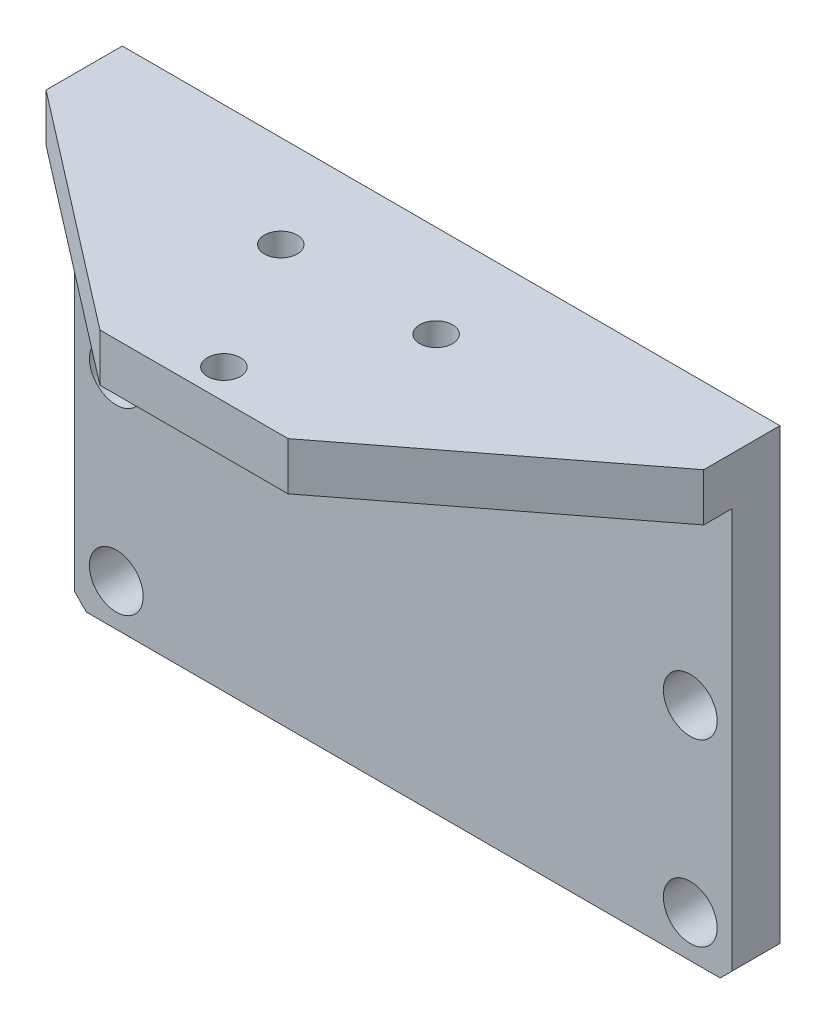
from build123d import *

# Parameters (mm, degrees)
SKETCH_1_W              = 110
SKETCH_1_H              = 77
EXTRUDE_1_DEPTH         = 8
SKETCH_2_W              = 110
SKETCH_2_H              = 8
EXTRUDE_3_DEPTH         = 43
SKETCH_4_OUTSIDE_W      = 140.198
SKETCH_4_OUTSIDE_H      = 73.198
CUT_EXTRUDE_1_DEPTH     = 43
HOLE_WIZARD_7_0_7_1_D   = 9
HOLE_WIZARD_5_5_5_5_2_D = 5.5
CHAMFER_1_SIZE          = 2


with BuildPart() as part:
    # 草图1 → 凸台-拉伸1 (new body)
    with BuildSketch(Plane.XY):
        Rectangle(SKETCH_1_W, SKETCH_1_H)
    extrude(amount=EXTRUDE_1_DEPTH)

    # 草图2 → 凸台-拉伸3 (add)
    with BuildSketch(Plane.XY):
        with Locations((0, 34.5)):
            Rectangle(SKETCH_2_W, SKETCH_2_H)
    extrude(amount=EXTRUDE_3_DEPTH)

    # 草图4 outside → 切除-拉伸1 (cut)
    with BuildSketch(Plane(origin=(0, 38.5, 0), x_dir=(1, 0, 0), z_dir=(0, 1, 0))):
        with Locations((0, -21.5)):
            Rectangle(SKETCH_4_OUTSIDE_W, SKETCH_4_OUTSIDE_H)
        Polygon((-55, 0), (55, 0), (55, -12.75), (15.74, -43), (-15.74, -43), (-55, -12.75), align=None, mode=Mode.SUBTRACT)
    extrude(amount=-CUT_EXTRUDE_1_DEPTH, mode=Mode.SUBTRACT)

    # Ø7.0 (7) 直径孔1 (through all)
    with Locations(Plane.XY.offset(8)):
        with Locations((-48, -31.5), (48, -31.5), (48, -1.5), (-48, -1.5)):
            Hole(HOLE_WIZARD_7_0_7_1_D / 2)

    # Ø5.5 (5.5) 直径孔2 (through all)
    with Locations(Plane(origin=(0, 38.5, 0), x_dir=(1, 0, 0), z_dir=(0, 1, 0))):
        with Locations((-12.990381057, -15.5), (12.990381057, -15.5), (0, -38)):
            Hole(HOLE_WIZARD_5_5_5_5_2_D / 2)

    # 倒角1
    chamfer_1_edges = [part.edges().sort_by_distance(p)[0] for p in [
        (55, -38.5, 4),
        (-55, -38.5, 4),
    ]]
    chamfer(chamfer_1_edges, length=CHAMFER_1_SIZE)


solid = part.part
